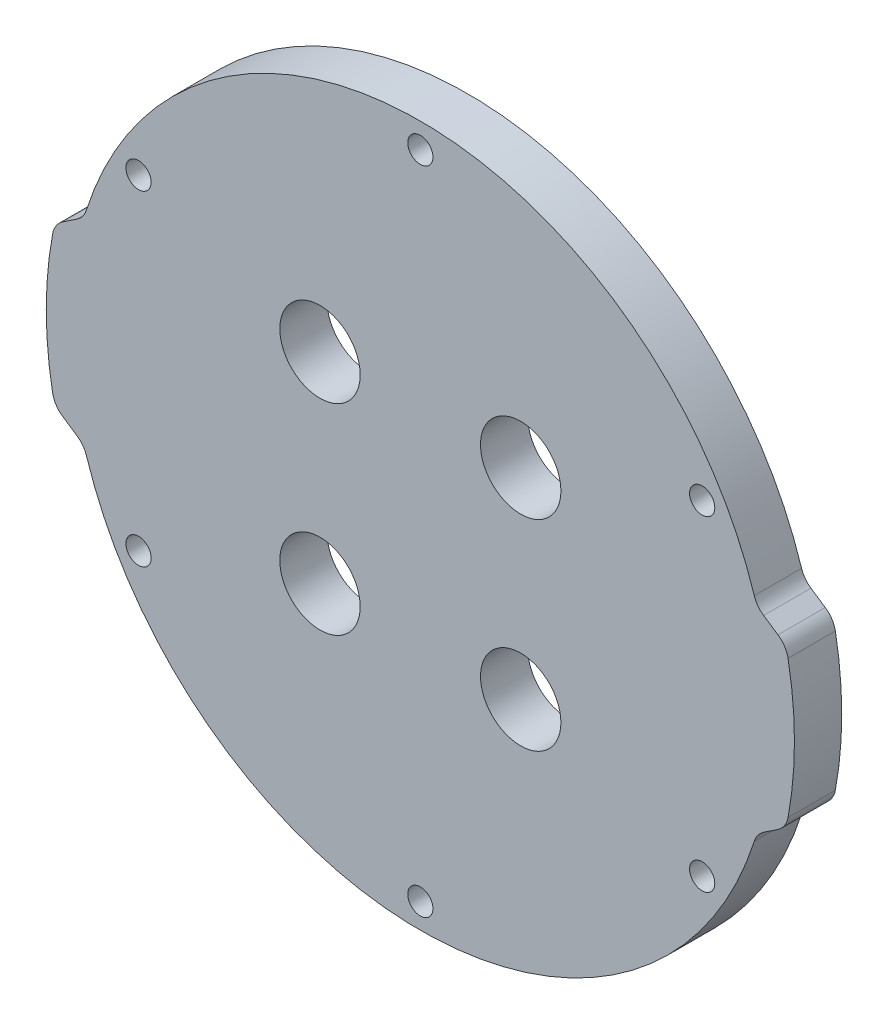
from build123d import *

# Parameters (mm, degrees)
SKETCH1_R           = 1.6
SKETCH1_R_2         = 5.1
BOSS_EXTRUDE1_DEPTH = 6


with BuildPart() as part:
    # Sketch1 → Boss-Extrude1 (new body)
    with BuildSketch(Plane.XY):
        with BuildLine():
            Line((-45.309203126, -10.68796842), (-43.492395524, -11.905920573))
            ThreePointArc((-43.492395524, -11.905920573), (-42.764262434, -12.595973377), (-42.304336877, -13.487499682))
            ThreePointArc((-42.304336877, -13.487499682), (0.05, -44.45), (42.404336877, -13.487499682))
            ThreePointArc((42.404336877, -13.487499682), (42.864262434, -12.595973377), (43.592395524, -11.905920573))
            Line((43.592395524, -11.905920573), (45.409203126, -10.68796842))
            ThreePointArc((45.409203126, -10.68796842), (46.243586183, -9.847021456), (46.68737785, -8.748642725))
            ThreePointArc((46.68737785, -8.748642725), (47.5, 0), (46.68737785, 8.748642725))
            ThreePointArc((46.68737785, 8.748642725), (46.243586183, 9.847021456), (45.409203126, 10.68796842))
            Line((45.409203126, 10.68796842), (43.592395524, 11.905920573))
            ThreePointArc((43.592395524, 11.905920573), (42.864262434, 12.595973377), (42.404336877, 13.487499682))
            ThreePointArc((42.404336877, 13.487499682), (0.05, 44.45), (-42.304336877, 13.487499682))
            ThreePointArc((-42.304336877, 13.487499682), (-42.764262434, 12.595973377), (-43.492395524, 11.905920573))
            Line((-43.492395524, 11.905920573), (-45.309203126, 10.68796842))
            ThreePointArc((-45.309203126, 10.68796842), (-46.143586183, 9.847021456), (-46.58737785, 8.748642725))
            ThreePointArc((-46.58737785, 8.748642725), (-47.4, 0), (-46.58737785, -8.748642725))
            ThreePointArc((-46.58737785, -8.748642725), (-46.143586183, -9.847021456), (-45.309203126, -10.68796842))
        make_face()
        with Locations((-35.695198541, 20.6375)):
            Circle(SKETCH1_R, mode=Mode.SUBTRACT)
        with Locations((-35.695198541, -20.6375)):
            Circle(SKETCH1_R, mode=Mode.SUBTRACT)
        with Locations((35.795198541, -20.6375)):
            Circle(SKETCH1_R, mode=Mode.SUBTRACT)
        with Locations((35.795198541, 20.6375)):
            Circle(SKETCH1_R, mode=Mode.SUBTRACT)
        with Locations((12.777922061, 12.727922061)):
            Circle(SKETCH1_R_2, mode=Mode.SUBTRACT)
        with Locations((12.777922061, -12.727922061)):
            Circle(SKETCH1_R_2, mode=Mode.SUBTRACT)
        with Locations((-12.677922061, -12.727922061)):
            Circle(SKETCH1_R_2, mode=Mode.SUBTRACT)
        with Locations((-12.677922061, 12.727922061)):
            Circle(SKETCH1_R_2, mode=Mode.SUBTRACT)
        with Locations((0.05, -41.275)):
            Circle(SKETCH1_R, mode=Mode.SUBTRACT)
        with Locations((0.05, 41.275)):
            Circle(SKETCH1_R, mode=Mode.SUBTRACT)
    extrude(amount=BOSS_EXTRUDE1_DEPTH)


solid = part.part
